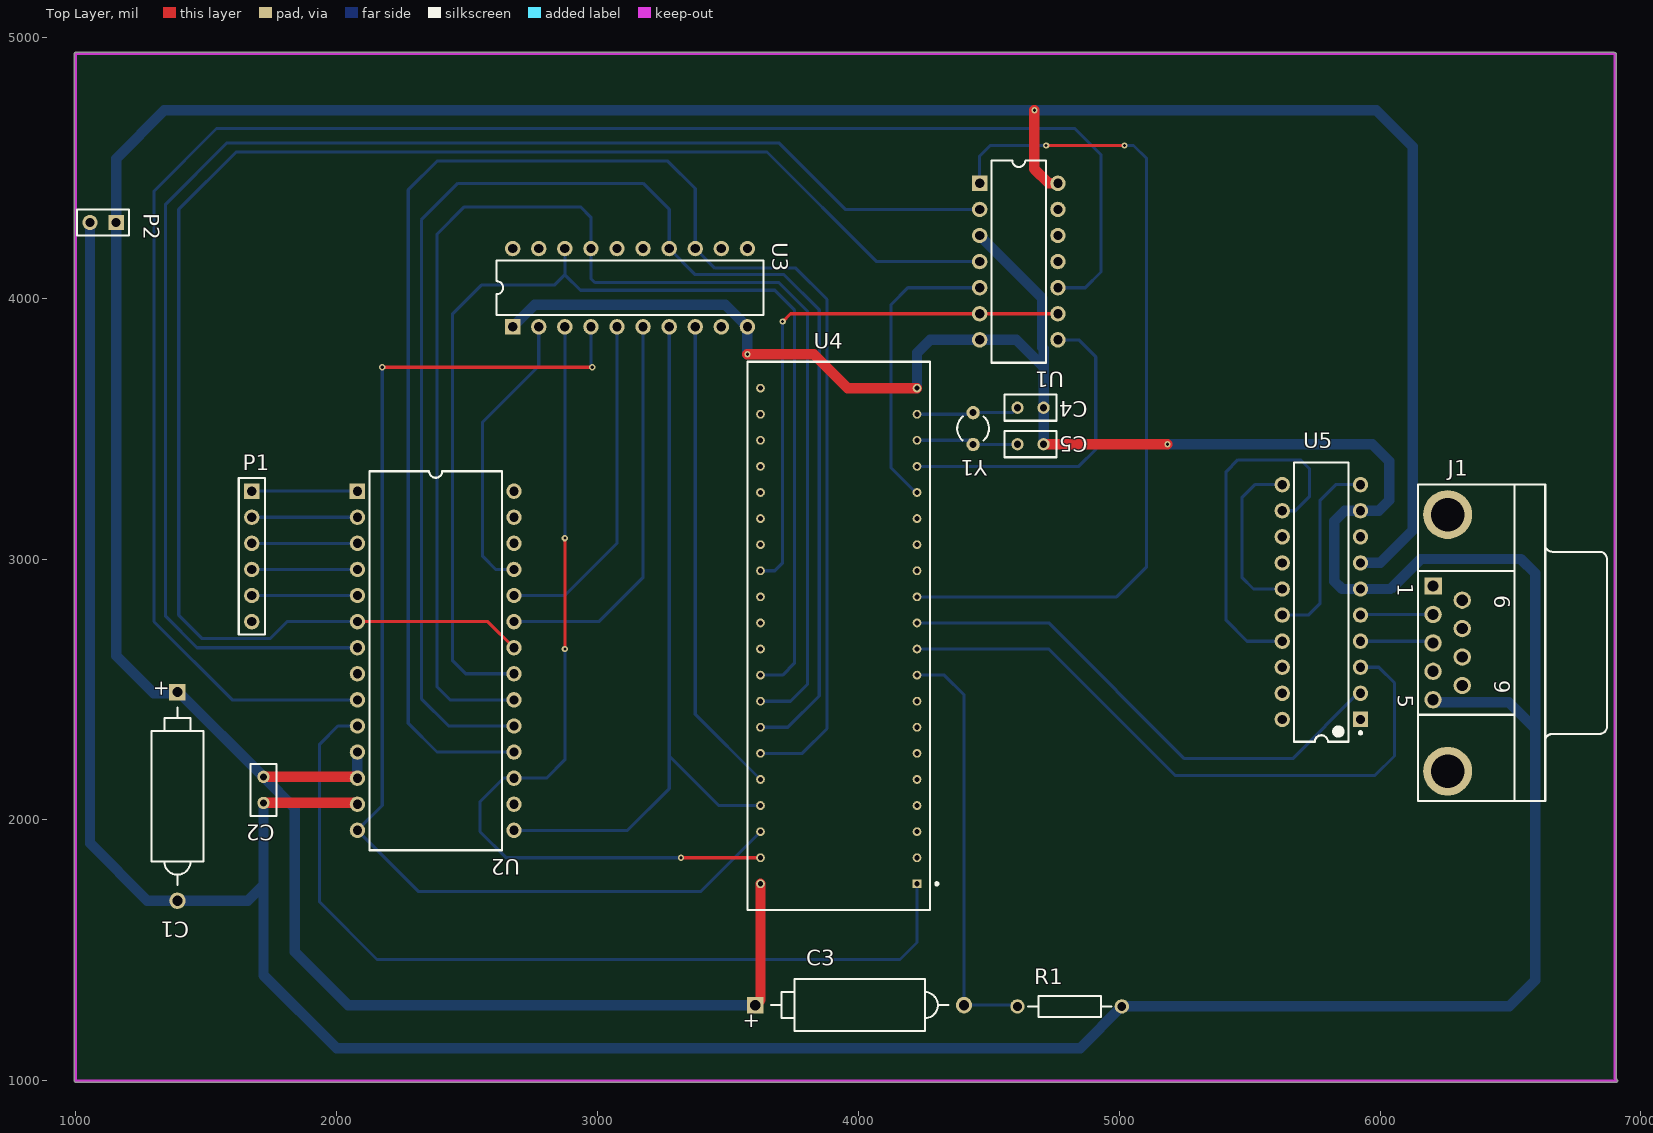
[diagram p0: Top Layer view]
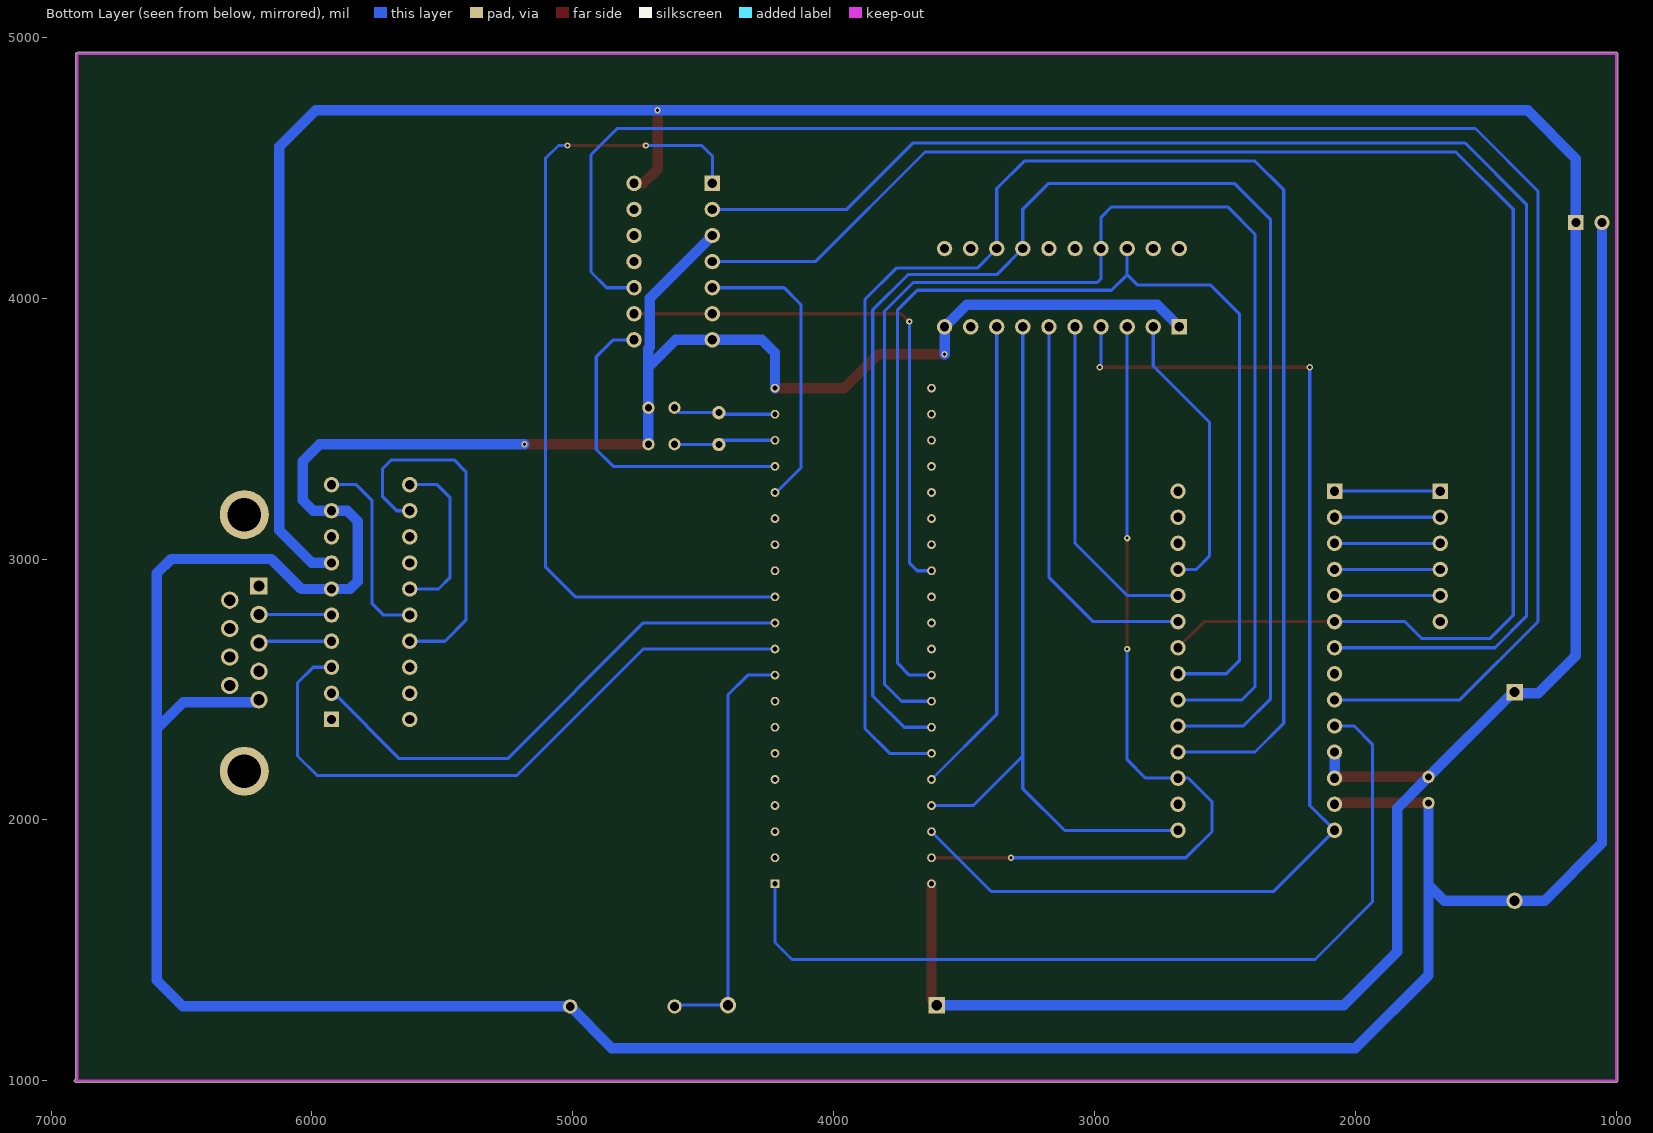
[diagram p1: Bottom Layer view, seen from below]
# Altium PCB MISC80520.PcbDoc
Units mil, origin at the board's own origin, x right, y up, seen from the top; angles counter-clockwise.
Board outline 5915.54 x 3947.04 mil, 2 copper layers (Top Layer, Bottom Layer); 15 components, 37 nets, 155 pads, 11 vias.

## Layer stack, top to bottom (the 12.6 mil dielectric is the usual default, probably not edited)
Top Solder: solder mask 0.4, Solder Resist, Dk 3.5
Top Layer: signal copper 1.4
Dielectric 1: dielectric 12.6, FR-4, Dk 4.8
Bottom Layer: signal copper 1.4
Bottom Solder: solder mask 0.4, Solder Resist, Dk 3.5

## Board outline
1000,994.99 cw(c1000,1000) 994.99,1000 994.99,4937.01 cw(c1000,4937.01) 1000,4942.02 6895.15,4942.02 cw(c6895.15,4937.01) 6899.21,4939.95 cw(c6900,4935) 6905.02,4935 6905.02,1013.31 ccw(c6918.82,1013.31) 6909.06,1003.55 cw(c6905.51,1000) 6910.53,1000 cw(c6905.51,1000) 6905.51,994.99

## Design rules (kind name [scope] priority, off if disabled: settings)
Clearance [All] p1: gap=10
HoleSize [All] p1: absolutevalues=TRUE maxlimit=3937.01 minlimit=1 maxpercent=80.000 minpercent=20.000
MinimumSolderMaskSliver [All] p1: minsoldermaskwidth=0
PolygonConnect [All] p1: connectstyle=Relief reliefconductorwidth=10 reliefentries=4 polygonreliefangle="90 Angle" airgapwidth=10
RoutingVias [All] p1: holewidth=28 width=50 viastyle="Through Hole" minholewidth=28 minwidth=50 maxholewidth=28 maxwidth=50
SilkToSilkClearance [All] p1: silktosilkclearance=0
SilkToSolderMaskClearance [IsPad] p1: minsilkscreentomaskgap=0 clearancetoexposedcopper=TRUE
SolderMaskExpansion [All] p1: expansion=4
Width [All] p1: maxlimit=40 minlimit=12 preferedwidth=20
26 further rules are at their usual default settings.

## Components (designator, comment, footprint, x,y, rotation, side; value= is the part's Value field where it differs from the comment)
C1 "10UF" POLAR0.8 1390,2090 r90 top
C2 "104" RAD-0.1 1720,2115 r270 top
C3 "10UF" POLAR0.8 4005,1290 r180 top
C4 "104" RAD-0.1 4660,3580 r180 top
C5 "104" RAD-0.1 4660,3440 r0 top
J1 "D Connector 9" DSUB1.385-2H9 6633.11,2678.58 r270 top
P1 "Header 6" HDR1X6 1675,3260 r270 top
P2 "Header 2" HDR1X2 1155,4290 r180 top
R1 "10K" AXIAL-0.4 4810,1285 r180 top
U1 "SN74LS02N" N014 4615,4140 r270 top
U2 "ADC0809CCN" N28B 2380,2610 r270 top
U3 "DM54S373J" J20A 3125,4040 r0 top
U4 "DS5000T-32-16" ENDIP40A 3925,2705 r90 top
U5 "MAX233AEPP" PP20 5775,2835 r180 top
Y1 "XTAL" R38 4440,3500 r180 top

## Footprints (in the part's own frame and the unit in brackets; to place one, negate y for a bottom-side part, rotate by r counter-clockwise, add the part's x,y. Pads: shape width x height; smd on the part's side, far side on the other; paste and mask are expansions set on the pad)
AXIAL-0.4 [mm] "Axial Device, Thru-Hole; 2 Leads; 0.4 in Pin Spacing"
  round 1.4 hole 0.85: 1(-5.08,0) 2(5.08,0)
  silkscreen extent -4.06,-1.02 4.06,1.02
DSUB1.385-2H9 [mm] "Connector; D Subminiature; 9 Position; Right Angle; Pitch 1.385 mm"
  rect 1.69x1.69 hole 1.09: 1(-5.54,-10.92)
  round 1.69 hole 1.09: 2(-2.77,-10.92) 3(0,-10.92) 4(2.77,-10.92) 5(5.54,-10.92) 6(-4.155,-8.08) 7(-1.385,-8.08) 8(1.385,-8.08) 9(4.155,-8.08)
  round 4.76 hole 3.26: 10(-12.495,-9.5) 11(12.495,-9.5)
  silkscreen extent -15.4,-12.4 15.4,6
ENDIP40A [mm] "DIP; 40 Rectangular Pins; Row Space 15.24 mm; Pitch 2.54 mm"
  rect 0.85x0.85 hole 0.5: 1(-24.13,-7.62)
  round 0.85 hole 0.5: 2(-21.59,-7.62) 3(-19.05,-7.62) 4(-16.51,-7.62) 5(-13.97,-7.62) 6(-11.43,-7.62) 7(-8.89,-7.62) 8(-6.35,-7.62) 9(-3.81,-7.62) 10(-1.27,-7.62) 11(1.27,-7.62) 12(3.81,-7.62) 13(6.35,-7.62) 14(8.89,-7.62) 15(11.43,-7.62) 16(13.97,-7.62) 17(16.51,-7.62) 18(19.05,-7.62) 19(21.59,-7.62) 20(24.13,-7.62) 21(24.13,7.62) 22(21.59,7.62) 23(19.05,7.62) 24(16.51,7.62) 25(13.97,7.62) 26(11.43,7.62) 27(8.89,7.62) 28(6.35,7.62) 29(3.81,7.62) 30(1.27,7.62) 31(-1.27,7.62) 32(-3.81,7.62) 33(-6.35,7.62) 34(-8.89,7.62) 35(-11.43,7.62) 36(-13.97,7.62) 37(-16.51,7.62) 38(-19.05,7.62) 39(-21.59,7.62) 40(-24.13,7.62)
  silkscreen extent -26.7,-9.68 26.7,8.9
HDR1X2 [mm] "Connector; Header; 2 Position"
  rect 1.5x1.5 hole 0.9: 1(0,0)
  round 1.5 hole 0.9: 2(2.54,0)
  silkscreen extent -1.27,-1.27 3.81,1.27
HDR1X6 [mm] "Connector; Header; 6 Position"
  rect 1.5x1.5 hole 0.9: 1(0,0)
  round 1.5 hole 0.9: 2(2.54,0) 3(5.08,0) 4(7.62,0) 5(10.16,0) 6(12.7,0)
  silkscreen extent -1.27,-1.27 13.97,1.27
J20A [mm] "DIP; 20 Leads; Row Spacing 7.62 mm; Pitch 2.54 mm"
  rect 1.5x1.5 hole 0.9: 1(-11.43,-3.81)
  round 1.5 hole 0.9: 2(-8.89,-3.81) 3(-6.35,-3.81) 4(-3.81,-3.81) 5(-1.27,-3.81) 6(1.27,-3.81) 7(3.81,-3.81) 8(6.35,-3.81) 9(8.89,-3.81) 10(11.43,-3.81) 11(11.43,3.81) 12(8.89,3.81) 13(6.35,3.81) 14(3.81,3.81) 15(1.27,3.81) 16(-1.27,3.81) 17(-3.81,3.81) 18(-6.35,3.81) 19(-8.89,3.81) 20(-11.43,3.81)
  silkscreen extent -13,-2.65 13,2.65
N014 [mm] "DIP; 14 Leads; Row Spacing 7.62 mm; Pitch 2.54 mm"
  rect 1.5x1.5 hole 0.9: 1(-7.62,-3.81)
  round 1.5 hole 0.9: 2(-5.08,-3.81) 3(-2.54,-3.81) 4(0,-3.81) 5(2.54,-3.81) 6(5.08,-3.81) 7(7.62,-3.81) 8(7.62,3.81) 9(5.08,3.81) 10(2.54,3.81) 11(0,3.81) 12(-2.54,3.81) 13(-5.08,3.81) 14(-7.62,3.81)
  silkscreen extent -9.85,-2.65 9.85,2.65
N28B [mm] "DIP; 28 Leads; Row Spacing 15.24 mm; Pitch 2.54 mm"
  rect 1.5x1.5 hole 0.9: 1(-16.51,-7.62)
  round 1.5 hole 0.9: 2(-13.97,-7.62) 3(-11.43,-7.62) 4(-8.89,-7.62) 5(-6.35,-7.62) 6(-3.81,-7.62) 7(-1.27,-7.62) 8(1.27,-7.62) 9(3.81,-7.62) 10(6.35,-7.62) 11(8.89,-7.62) 12(11.43,-7.62) 13(13.97,-7.62) 14(16.51,-7.62) 15(16.51,7.62) 16(13.97,7.62) 17(11.43,7.62) 18(8.89,7.62) 19(6.35,7.62) 20(3.81,7.62) 21(1.27,7.62) 22(-1.27,7.62) 23(-3.81,7.62) 24(-6.35,7.62) 25(-8.89,7.62) 26(-11.43,7.62) 27(-13.97,7.62) 28(-16.51,7.62)
  silkscreen extent -18.45,-6.45 18.45,6.45
POLAR0.8 [mm] "Polarized Capacitor; 2 Leads"
  rect 1.6x1.6 hole 1: 1(10.16,0)
  round 1.6 hole 1: 2(-10.16,0)
  silkscreen extent -8.64,-2.54 8.64,2.54
PP20 [mm] "DIP, 20-Leads, Row Spacing 7.62mm, Pitch 2.54mm, Body 26.16x7.24mm"
  rect 1.5x1.5 hole 0.9: 1(-3.81,11.43)
  round 1.5 hole 0.9: 2(-3.81,8.89) 3(-3.81,6.35) 4(-3.81,3.81) 5(-3.81,1.27) 6(-3.81,-1.27) 7(-3.81,-3.81) 8(-3.81,-6.35) 9(-3.81,-8.89) 10(-3.81,-11.43) 11(3.81,-11.43) 12(3.81,-8.89) 13(3.81,-6.35) 14(3.81,-3.81) 15(3.81,-1.27) 16(3.81,1.27) 17(3.81,3.81) 18(3.81,6.35) 19(3.81,8.89) 20(3.81,11.43)
  silkscreen extent -3.94,-13.6 2.65,13.6, body extent -3.3,-13.57 3.3,13.57, height 4.58
R38 [mm] "Crystal, Thru-Hole; 2 Leads; Body 3.1 x 8.2 mm (Dia.xH)"
  round 1.3 hole 0.7: 1(0,1.55) 2(0,-1.55)
  silkscreen extent -1.55,-1.19 1.55,1.17
RAD-0.1 [mm] "Radial Cap, Thru-Hole; 2 Leads; 0.1 in Pin Spacing"
  round 1.2 hole 0.7: 1(-1.27,0) 2(1.27,0)
  silkscreen extent -2.54,-1.27 2.54,1.27

## Part data
C1 C3: library part "Cap Pol2", "Polarized Capacitor (Axial)"
C2 C4 C5: library part Cap, "Capacitor"
J1: "Receptacle Assembly, 9 Position, Right Angle"
P1: "Header, 6-Pin"
P2: "Header, 2-Pin"
R1: library part Res2, "Resistor"
U1: "Quadruple 2-Input Positive-NOR Gate"
U2: "8-Bit uP-Compatible A/D Converter with 8-Channel Multiplexer"
U3: "Octal D-Type Transparent Latch and Edge-Triggered Flip-Flop"
U4: "Soft Microcontroller"
U5: "+5V-Powered, Multichannel RS-232 Driver/Receiver"
Y1: "Crystal Oscillator"

## Via types
v1: diameter 24, hole 12, Top Layer to Bottom Layer, 11 vias

## Nets (pads, with @x,y where several pads share a name; then routed paths per layer and width w, separated by ;. In a path a pad name is that pad's centre, name@x,y a point inside that pad or via, vN(x,y) a via of type N, cw(c..) or ccw(c..) an arc to the next point about the centre after c; other vN are vias at no path point)
A: U2.25 U3.2 | length 1109.8
  Bottom Layer w12: U2.25 2610,2960 2560,3010 2560,3525 2775,3740 U3.2
AD_CLK: U2.10 U4.1 | length 3412
  Bottom Layer w12: U2.10 2005,2360 1935,2290 1935,1685 2155,1465 4160,1465 4225,1530 U4.1
ALE: U3.11
B: U2.24 U3.5 | length 1307.8
  Bottom Layer w12: U2.24 2875,2860 3075,3060 U3.5
C: U2.23 U3.6 | length 1525.4
  Bottom Layer w12: U2.23 3005,2760 3175,2930 U3.6
EOC: U1.2 U2.7 | length 5687.7
  Bottom Layer w12: U2.7 1465,2660 1345,2780 1345,4360 1580,4595 3695,4595 3950,4340 U1.2
GND: C1.2 C2.2 C4.1 C5.2 J1.5 P2.2 R1.1 U1.3 U1.7 U2.13 U3.1 U3.10 U4.20 U5.6 U5.9 | length 17477.3
  Top Layer w40: C2.2 2075,2065 U2.13 ; v1(3575,3785) 3830,3785 3960,3655 U4.20 ; C5.2 v1(5185,3440)
  Bottom Layer w40: P2.2 1055,1910 1275,1690 C1.2 1660,1690 1720,1750 ; C2.2 1720,1750 ; U3.1 2760,3975 3490,3975 U3.10 v1(3575,3785) ; U4.20 4225,3790 4275,3840 U1.7 4605,3840 4710,3735 ; U1.3 4705.47,3999.53 4705.47,3810.82 4710,3806.29 4710,3735 ; C5.2 C4.1 4710,3735 ; v1(5185,3440) 5970,3440 6035,3375 6035,3225 5995,3185 U5.9 5865,3185 5825,3145 5825,2915 5855,2885 U5.6 6040,2885 6155,3000 6540,3000 6595,2945 6595,2350 ; J1.5 6203.19,2451.73 6493.27,2451.73 6595,2350 ; 1720,1750 1720,1405 2000,1125 4850,1125 R1.1 6495,1285 6595,1385 6595,2350
INT0: U1.1 U4.12 | length 3274.9
  Top Layer w12: v1(4720,4585) v1(5020,4585)
  Bottom Layer w12: U4.12 4990,2855 5105,2970 5105,4535 5055,4585 v1(5020,4585) ; U1.1 4465,4545 4505,4585 v1(4720,4585)
NetC3_2: C3.2 R1.2 U4.9 | length 1608.1
  Bottom Layer w12: U4.9 4330,2555 4405,2480 C3.2 4605,1290 R1.2
NetC4_2: C4.2 U4.19 Y1.2 | length 395.4
  Bottom Layer w12: U4.19 4433.98,3555 Y1.2 4591.02,3561.02 C4.2
NetC5_1: C5.1 U4.18 Y1.1 | length 392.1
  Bottom Layer w12: U4.18 4423.98,3455 Y1.1 4608.98,3438.98 C5.1
NetJ1_2: J1.2 U5.5 | length 279.3
  Bottom Layer w12: U5.5 5927.64,2787.64 J1.2
NetJ1_3: J1.3 U5.4 | length 280.8
  Bottom Layer w12: U5.4 6196.77,2685 J1.3
NetP1_1: P1.1 U2.1 | length 405
  Bottom Layer w12: P1.1 U2.1
NetP1_2: P1.2 U2.2 | length 405
  Bottom Layer w12: P1.2 U2.2
NetP1_3: P1.3 U2.3 | length 405
  Bottom Layer w12: P1.3 U2.3
NetP1_4: P1.4 U2.4 | length 405
  Bottom Layer w12: P1.4 U2.4
NetP1_5: P1.5 U2.5 | length 405
  Bottom Layer w12: P1.5 U2.5
NetU5_10: U5.10 U5.16 | length 738.5
  Bottom Layer w12: U5.16 5725,2785 5770,2830 5770,3225 5830,3285 U5.10
NetU5_11: U5.11 U5.15 | length 654.4
  Bottom Layer w12: U5.15 5515,2885 5470,2930 5470,3235 5520,3285 U5.11
NetU5_12: U5.12 U5.17 | length 1404.1
  Bottom Layer w12: U5.17 5490,2685 5410,2765 5410,3335 5455,3380 5695,3380 5730,3345 5730,3240 5675,3185 U5.12
OE: U1.10 U2.9 | length 6964.9
  Bottom Layer w12: U2.9 1600,2460 1300,2760 1300,4410 1540,4650 4830,4650 4930,4550 4930,4100 4870,4040 U1.10
P00: U2.17 U3.3 U4.39 | length 3282.7
  Top Layer w12: v1(2875,2655) v1(2875,3080) ; v1(3320,1855) U4.39
  Bottom Layer w12: v1(2875,2655) 2875,2230 2805,2160 U2.17 2640,2160 2550,2070 2550,1955 2650,1855 v1(3320,1855) ; v1(2875,3080) U3.3
P01: U2.14 U3.4 U4.38 | length 4521.1
  Top Layer w12: v1(2175,3735) v1(2980,3735)
  Bottom Layer w12: v1@2170,3740 v1(2175,3735) 2175,2055 U2.14 2315,1725 3395,1725 U4.38 ; U3.4 2975,3740 v1(2980,3735)
P02: U2.15 U3.7 U4.37 | length 2860
  Bottom Layer w12: U2.15 3115,1960 3275,2120 3275,2245 ; U3.7 3275,2245 ; U4.37 3465,2055 3275,2245
P03: U3.8 U4.36 | length 1838.6
  Bottom Layer w12: U3.8 3375,2405 U4.36
P04: U2.18 U3.13 U4.35 | length 6446.8
  Bottom Layer w12: U2.18 2385,2260 2275,2370 2275,4415 2385,4525 3270,4525 3375,4420 U3.13 3450,4115 3760,4115 3880,3995 3880,2350 3785,2255 U4.35 U4.35@3620,2260
P05: U2.19 U3.14 U4.34 | length 5867
  Bottom Layer w12: U2.19@2685,2355 U2.19 2430,2360 2325,2465 2325,4300 2465,4440 3175,4440 3275,4340 U3.14 3375,4090 3715,4090 3850,3955 3850,2475 3730,2355 U4.34
P06: U2.20 U3.17 U4.33 | length 5461.5
  Bottom Layer w12: U2.20 2435,2460 2385,2510 2385,4245 2490,4350 2935,4350 2975,4310 U3.17 2975,4075 2990,4060 3695,4060 3805,3950 3805,2520 3740,2455 U4.33 U4.33@3620,2460
P07: U2.21 U3.18 U4.32 | length 4624.5
  Bottom Layer w12: U2.21 2495,2560 2445,2610 2445,3940 2555,4050 2835,4050 2875,4090 ; U3.18 2875,4090 ; U4.32@3620,2560 U4.32 3710,2555 3755,2600 3755,3955 3680,4030 2935,4030 2875,4090
P27: U1.6 U1.9 U4.28 | length 2089.9
  Top Layer w12: v1(3710,3910) 3740,3940 U1.6 U1.9
  Bottom Layer w12: U4.28 3680,2955 3710,2985 v1(3710,3910)
RD: U1.8 U4.17 | length 1238.8
  Bottom Layer w12: U4.17 4845,3355 4910,3420 4910,3775 4845,3840 U1.8
RX: U4.10 U5.3 | length 2496.8
  Bottom Layer w12: U4.10 4730,2655 5215,2170 5980,2170 6055,2245 6055,2525 5995,2585 U5.3
START: U1.4 U2.6 U2.22 | length 6280.7
  Top Layer w12: U2.6 2580,2760 U2.22
  Bottom Layer w12: U2.6 1810,2760 1745,2695 1485,2695 1395,2785 1395,4340 1615,4560 3650,4560 4070,4140 U1.4
TX: U4.11 U5.2 | length 2018.9
  Bottom Layer w12: U4.11 4730,2755 5250,2235 5665,2235 5915,2485 U5.2
VCC: C1.1 C2.1 C3.1 P2.1 U1.14 U2.11 U2.12 U4.40 U5.7 | length 13335.9
  Top Layer w40: C2.1 2075,2165 U2.12 ; C3.1 3625,1310 U4.40 ; v1(4675,4720) 4675,4495 4730,4440 U1.14
  Bottom Layer w40: U2.12 U2.11 ; C3.1 2045,1290 1840,1495 1840,2045 C2.1 1395,2490 C1.1 1385,2485 1300,2485 1155,2630 P2.1 1155,4535 1340,4720 v1(4675,4720) 5985,4720 6125,4580 6125,3110 6000,2985 U5.7
WR: U1.5 U4.16 | length 1131.3
  Bottom Layer w12: U4.16 4220,3255 4125,3350 4125,3975 4190,4040 U1.5
pads on no net: J1.1 J1.4 J1.6 J1.7 J1.8 J1.9 J1.10 J1.11 P1.6 U1.11 U1.12 U1.13 U2.8 U2.16 U2.26 U2.27 U2.28 U3.9 U3.12 U3.15 U3.16 U3.19 U3.20 U4.2 U4.3 U4.4 U4.5 U4.6 U4.7 U4.8 U4.13 U4.14 U4.15 U4.21 U4.22 U4.23 U4.24 U4.25 U4.26 U4.27 U4.29 U4.30 U4.31 U5.1 U5.8 U5.13 U5.14 U5.18 U5.19 U5.20

## Keep-outs
Keep-Out Layer:
  lines w10: 6895.15,4937.01 1000,4937.01 1000,1000 6905.51,1000 cw(c6918.82,1013.31) 6900,1013.31 6900,4935